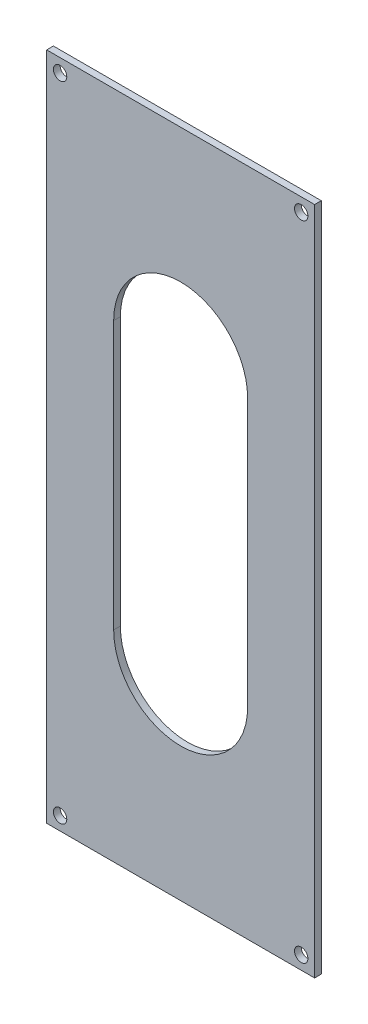
SolidWorks part; units mm, degrees
ref_plane "Front Plane" through (0, 0, 0) normal (0, 0, 1) x (1, 0, 0)
ref_plane "Top Plane" through (0, 0, 0) normal (0, 1, 0) x (1, 0, 0)
ref_plane "Right Plane" through (0, 0, 0) normal (1, 0, 0) x (0, 0, -1)
other "Configuration Table"
sketch "Sketch1" plane through (0, 0, 0) normal (0, 0, 1) x (1, 0, 0)
  line L1 (-200, -500) -> (200, -500)
  line L2 (-200, -500) -> (-200, 500)
  line L3 (-200, 500) -> (200, 500)
  line L4 (200, -500) -> (200, 500)
  line L5 (-200, -500) -> (200, 500) construction
  line L6 (-200, 500) -> (200, -500) construction
  point P0 (0, 0)
  dimension "D1" = 400
  dimension "D2" = 1000
extrude "Boss-Extrude1" add sketch "Sketch1" along normal blind 10
sketch "Sketch2" plane through (0, 0, 0) normal (0, 0, -1) x (-1, 0, 0)
  line L0 (0, 500) -> (0, -500) construction
  line L1 (-200, 500) -> (200, 500) construction
  line L2 (200, -500) -> (-200, -500) construction
  line L3 (-200, 0) -> (200, 0) construction
  line L4 (-200, -500) -> (-200, 500) construction
  line L5 (200, 500) -> (200, -500) construction
  circle A0 centre (-180, 480) radius 10
  circle A1 centre (180, 480) radius 10
  circle A2 centre (180, -480) radius 10
  circle A3 centre (-180, -480) radius 10
  dimension "D1" = 20
  dimension "D2" = 180
  dimension "D3" = 480
extrude "Cut-Extrude1" cut sketch "Sketch2" against normal blind 42
sketch "Sketch3" plane through (0, 0, 10) normal (0, 0, 1) x (1, 0, 0)
  line L0 (0, 500) -> (0, -500) construction
  line L1 (200, 500) -> (-200, 500) construction
  line L2 (-200, -500) -> (200, -500) construction
  line L3 (-200, 0) -> (200, 0) construction
  line L5 (-200, 500) -> (-200, -500) construction
  line L6 (200, -500) -> (200, 500) construction
  line L7 (0, 200) -> (0, -200) construction
  line L8 (100, 200) -> (100, -200)
  line L9 (-100, 200) -> (-100, -200)
  arc A0 (100, 200) -> (-100, 200) centre (0, 200) ccw
  arc A1 (-100, -200) -> (100, -200) centre (0, -200) ccw
  point P14 (0, 0)
  dimension "D3" = 100
  dimension "D1" = 200
  dimension "D2" = 200
extrude "Cut-Extrude2" cut sketch "Sketch3" against normal blind 20
